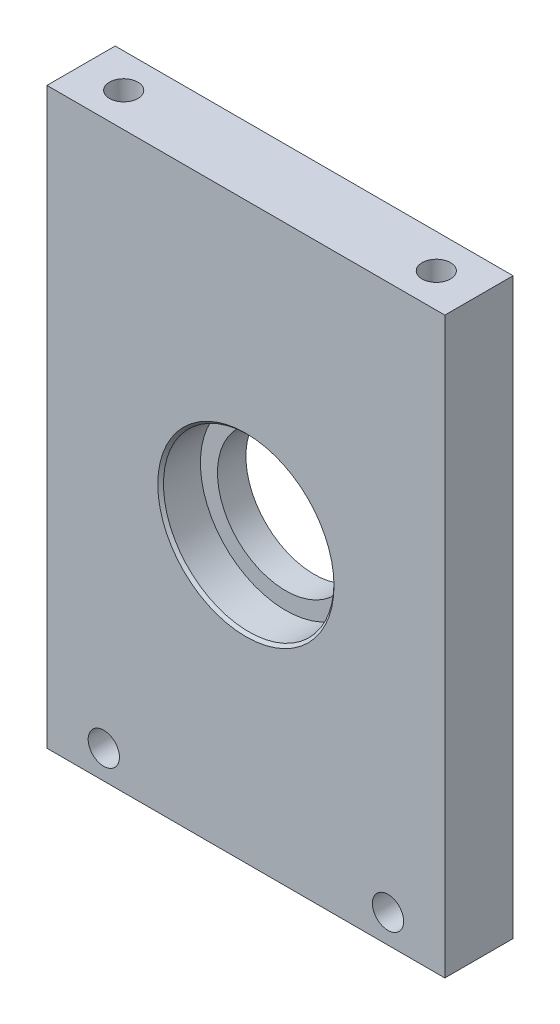
from build123d import *

# Parameters (mm, degrees)
SKETCH_1_W             = 70
SKETCH_1_H             = 101
EXTRUDE_1_DEPTH        = 12
SKETCH_2_R             = 15
CUT_EXTRUDE_1_DEPTH    = 7
SKETCH_3_R             = 12
CUT_EXTRUDE_2_DEPTH    = 124.085336251
CHAMFER_2_SIZE         = 0.5
HOLE_WIZARD_M6_1_D     = 5
HOLE_WIZARD_M6_1_DEPTH = 17
HOLE_WIZARD_M6_1_TIP   = 1.502151548
SKETCH_10_R            = 2.75
CUT_EXTRUDE_3_DEPTH    = 124.470644284


with BuildPart() as part:
    # 草图1 → 凸台-拉伸1 (new body)
    with BuildSketch(Plane.XY):
        with Locations((35, -50.5)):
            Rectangle(SKETCH_1_W, SKETCH_1_H)
    extrude(amount=EXTRUDE_1_DEPTH)

    # 草图2 → 切除-拉伸1 (cut)
    with BuildSketch(Plane.XY.offset(12)):
        with Locations((35, -51)):
            Circle(SKETCH_2_R)
    extrude(amount=-CUT_EXTRUDE_1_DEPTH, mode=Mode.SUBTRACT)

    # 草图3 → 切除-拉伸2 (cut, through all)
    with BuildSketch(Plane.XY.offset(5)):
        with Locations((35, -51)):
            Circle(SKETCH_3_R)
    extrude(amount=-CUT_EXTRUDE_2_DEPTH, mode=Mode.SUBTRACT)

    # 倒角2
    chamfer_2_edges = [part.edges().sort_by_distance(p)[0] for p in [
        (20, -51, 12),
    ]]
    chamfer(chamfer_2_edges, length=CHAMFER_2_SIZE)

    # M6 螺纹孔1
    with Locations(Plane(origin=(0, 0, 0), x_dir=(1, 0, 0), z_dir=(0, 1, 0))):
        with Locations((62.5, -6), (7.5, -6)):
            Hole(HOLE_WIZARD_M6_1_D / 2, depth=HOLE_WIZARD_M6_1_DEPTH)
            with Locations((0, 0, -(HOLE_WIZARD_M6_1_DEPTH + HOLE_WIZARD_M6_1_TIP / 2))):  # 118° drill point
                Cone(0, HOLE_WIZARD_M6_1_D / 2, HOLE_WIZARD_M6_1_TIP, mode=Mode.SUBTRACT)

    # 草图10 → 切除-拉伸3 (cut, through all)
    with BuildSketch(Plane(origin=(0, 0, 0), x_dir=(-1, 0, 0), z_dir=(0, 0, -1))):
        with Locations((-60, -96)):
            Circle(SKETCH_10_R)
        with Locations((-10, -96)):
            Circle(SKETCH_10_R)
    extrude(amount=-CUT_EXTRUDE_3_DEPTH, mode=Mode.SUBTRACT)


solid = part.part
